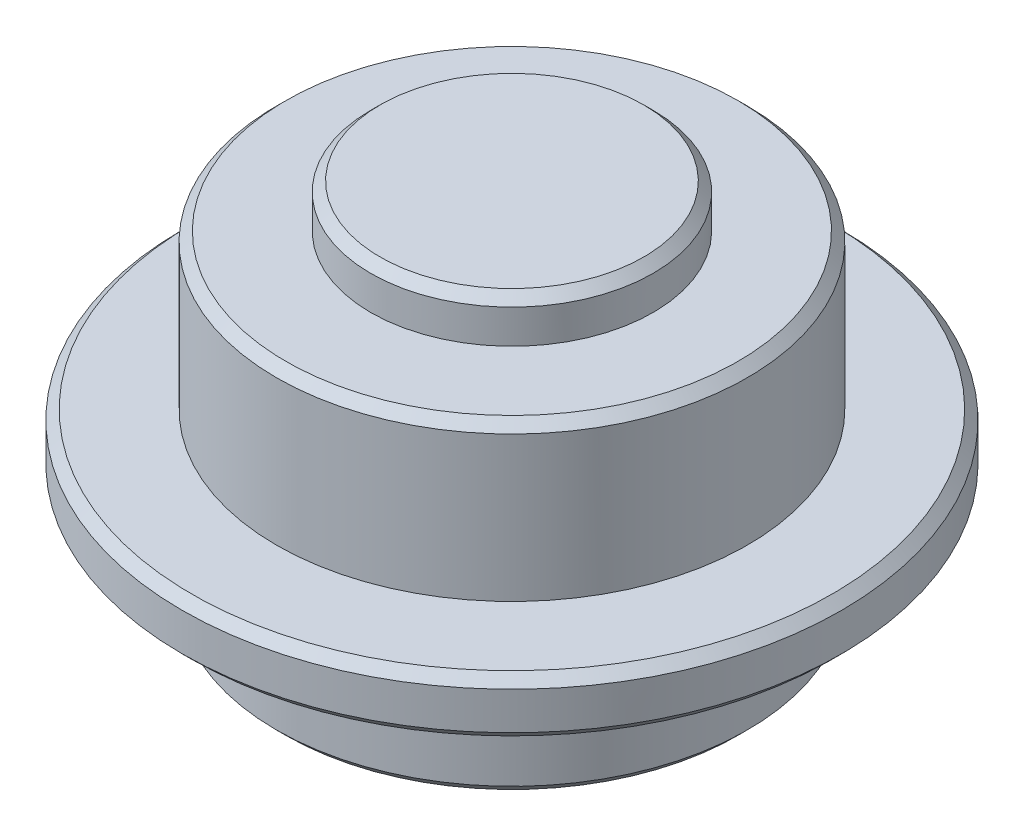
from build123d import *

# Parameters (mm, degrees)
CHAMFER1_SIZE = 0.5


with BuildPart() as part:
    # Sketch1 → Revolve1 (revolve)
    with BuildSketch(Plane.XY, mode=Mode.PRIVATE) as revolve1_sk:
        Polygon((380.5, -9.2), (380.5, -3.2), (385.5, -3.2), (385.5, -0.2), (380.5, -0.2), (380.5, 8), (375.5, 8), (375.5, 10.3), (368, 10.3), (368, -9.2), align=None)
    revolve(revolve1_sk.sketch.rotate(Axis((368, 10.3, 0), (0, -1, 0)), 90), axis=Axis((368, 10.3, 0), (0, -1, 0)))

    # Chamfer1
    chamfer1_edges = [part.edges().sort_by_distance(p)[0] for p in [
        (368, -0.2, -17.5),
        (368, -3.2, -17.5),
        (368, -9.2, -12.5),
        (368, 10.3, -7.5),
        (368, 8, -12.5),
    ]]
    chamfer(chamfer1_edges, length=CHAMFER1_SIZE)


solid = part.part
